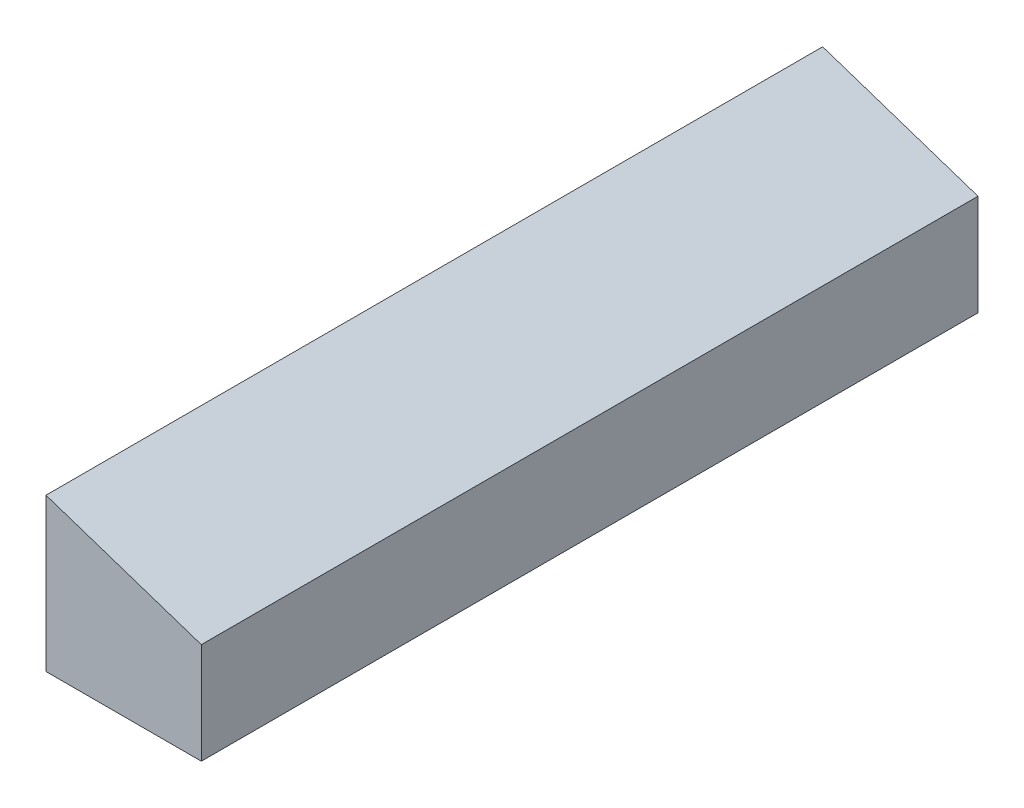
from build123d import *

# Parameters (mm, degrees)
BOSS_EXTRUDE1_DEPTH = 300
SHELL1_T            = -2
SKETCH2_W           = 120
SKETCH2_H           = 600
CUT_EXTRUDE1_DEPTH  = 2


with BuildPart() as part:
    # Sketch1 → Boss-Extrude1 (new, symmetric)
    with BuildSketch(Plane.XY):
        Polygon((0, 120), (120, 80), (120, 0), (0, 0), align=None)
    extrude(amount=BOSS_EXTRUDE1_DEPTH, both=True)

    # Shell1
    shell1_openings = [part.faces().sort_by_distance(p)[0] for p in [
        (0, 60, 0),
    ]]
    offset(amount=SHELL1_T, openings=shell1_openings, kind=Kind.INTERSECTION)

    # Sketch2 → Cut-Extrude1 (cut)
    with BuildSketch(Plane.XZ):
        with Locations((60, 0)):
            Rectangle(SKETCH2_W, SKETCH2_H)
    extrude(amount=-CUT_EXTRUDE1_DEPTH, mode=Mode.SUBTRACT)


solid = part.part
